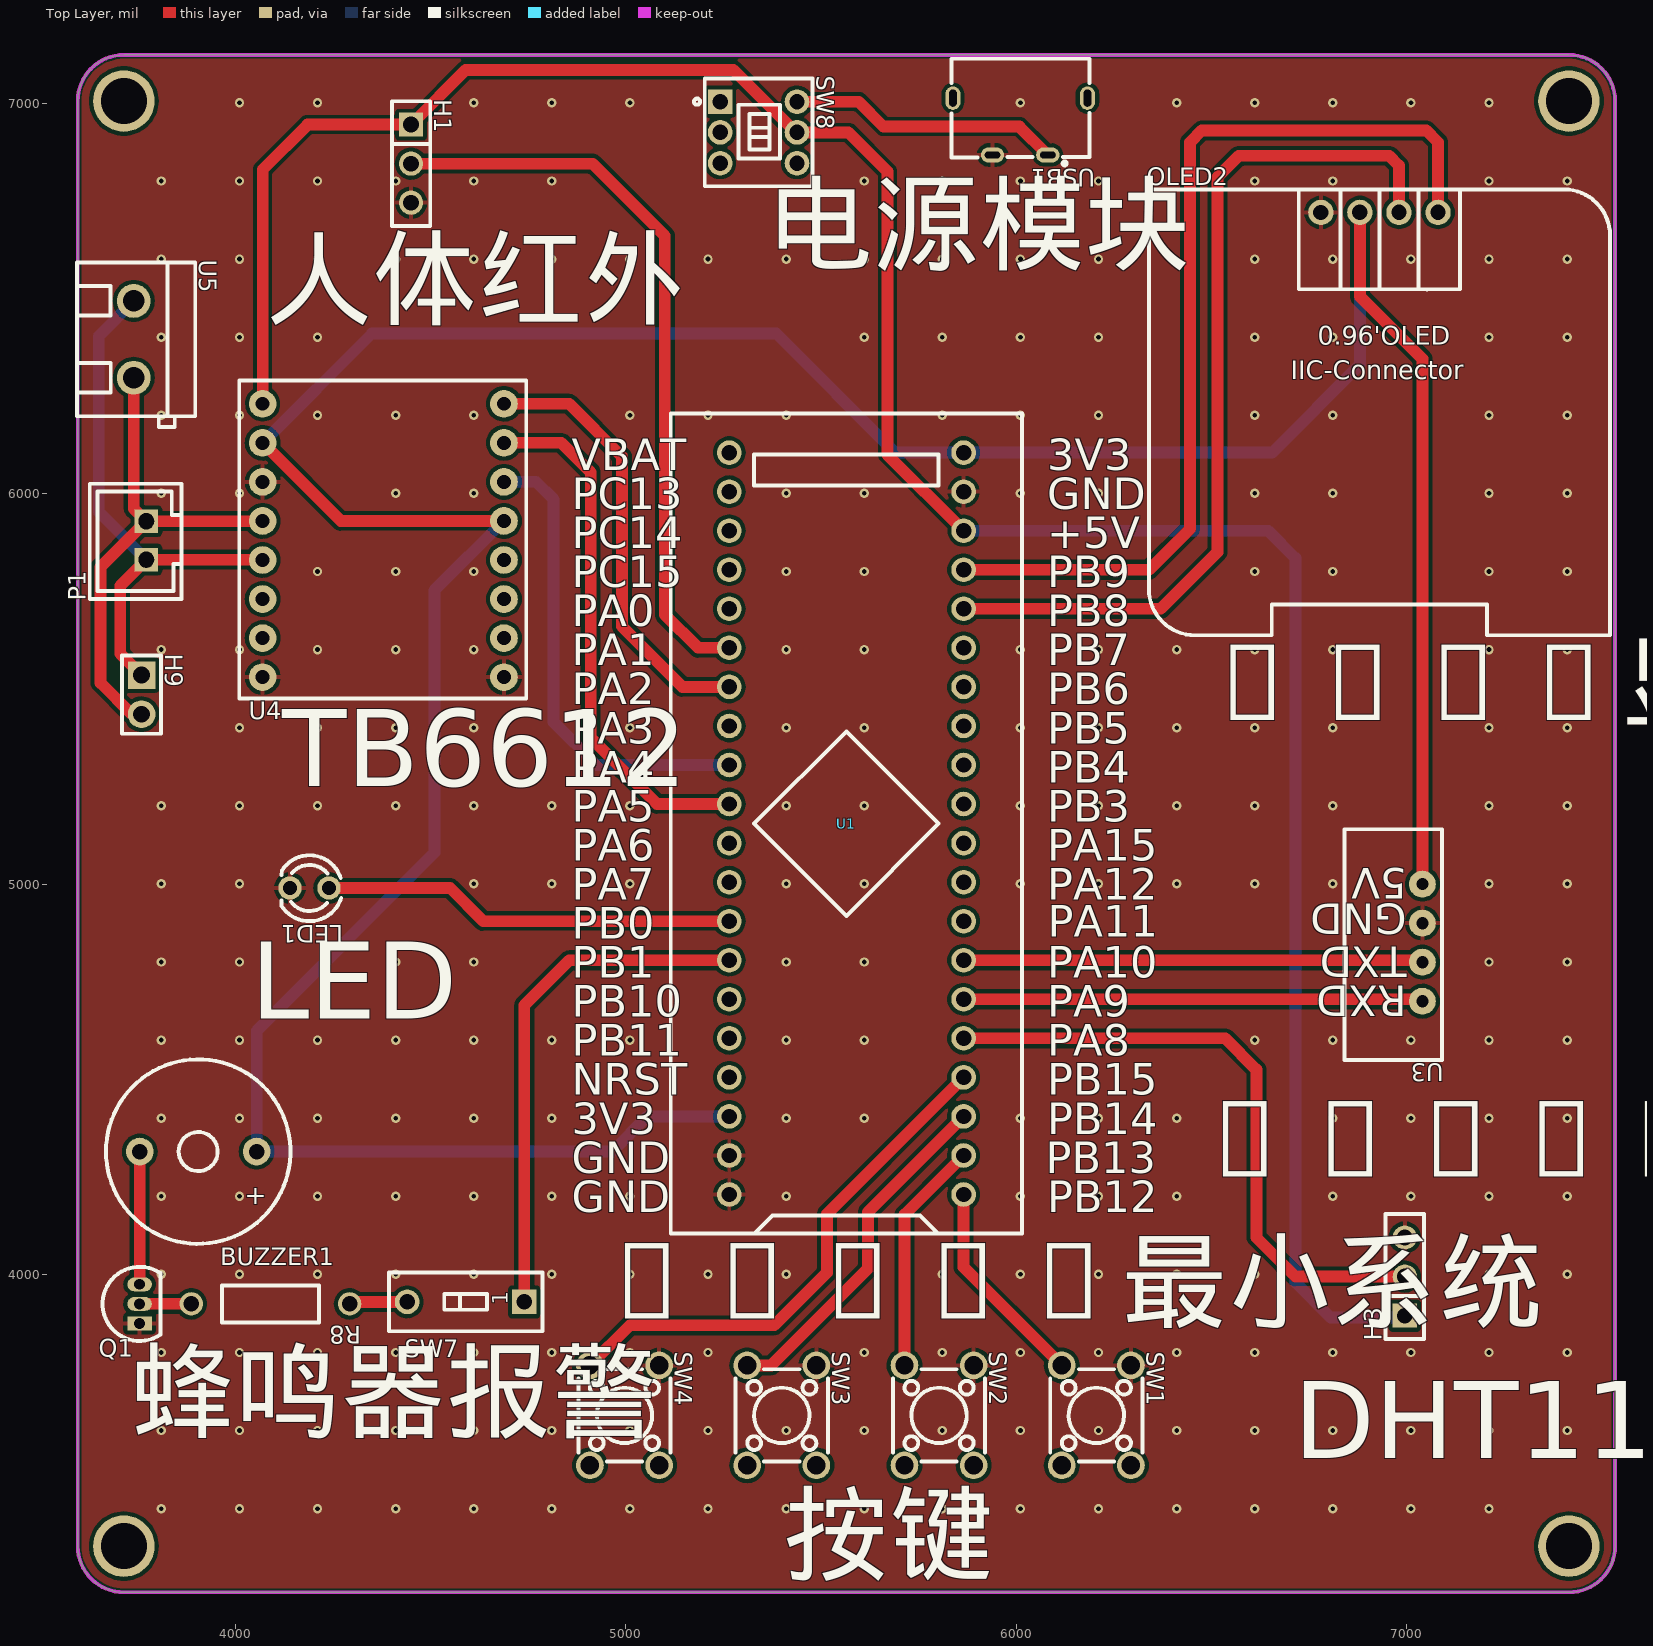
[diagram p0: Top Layer view]
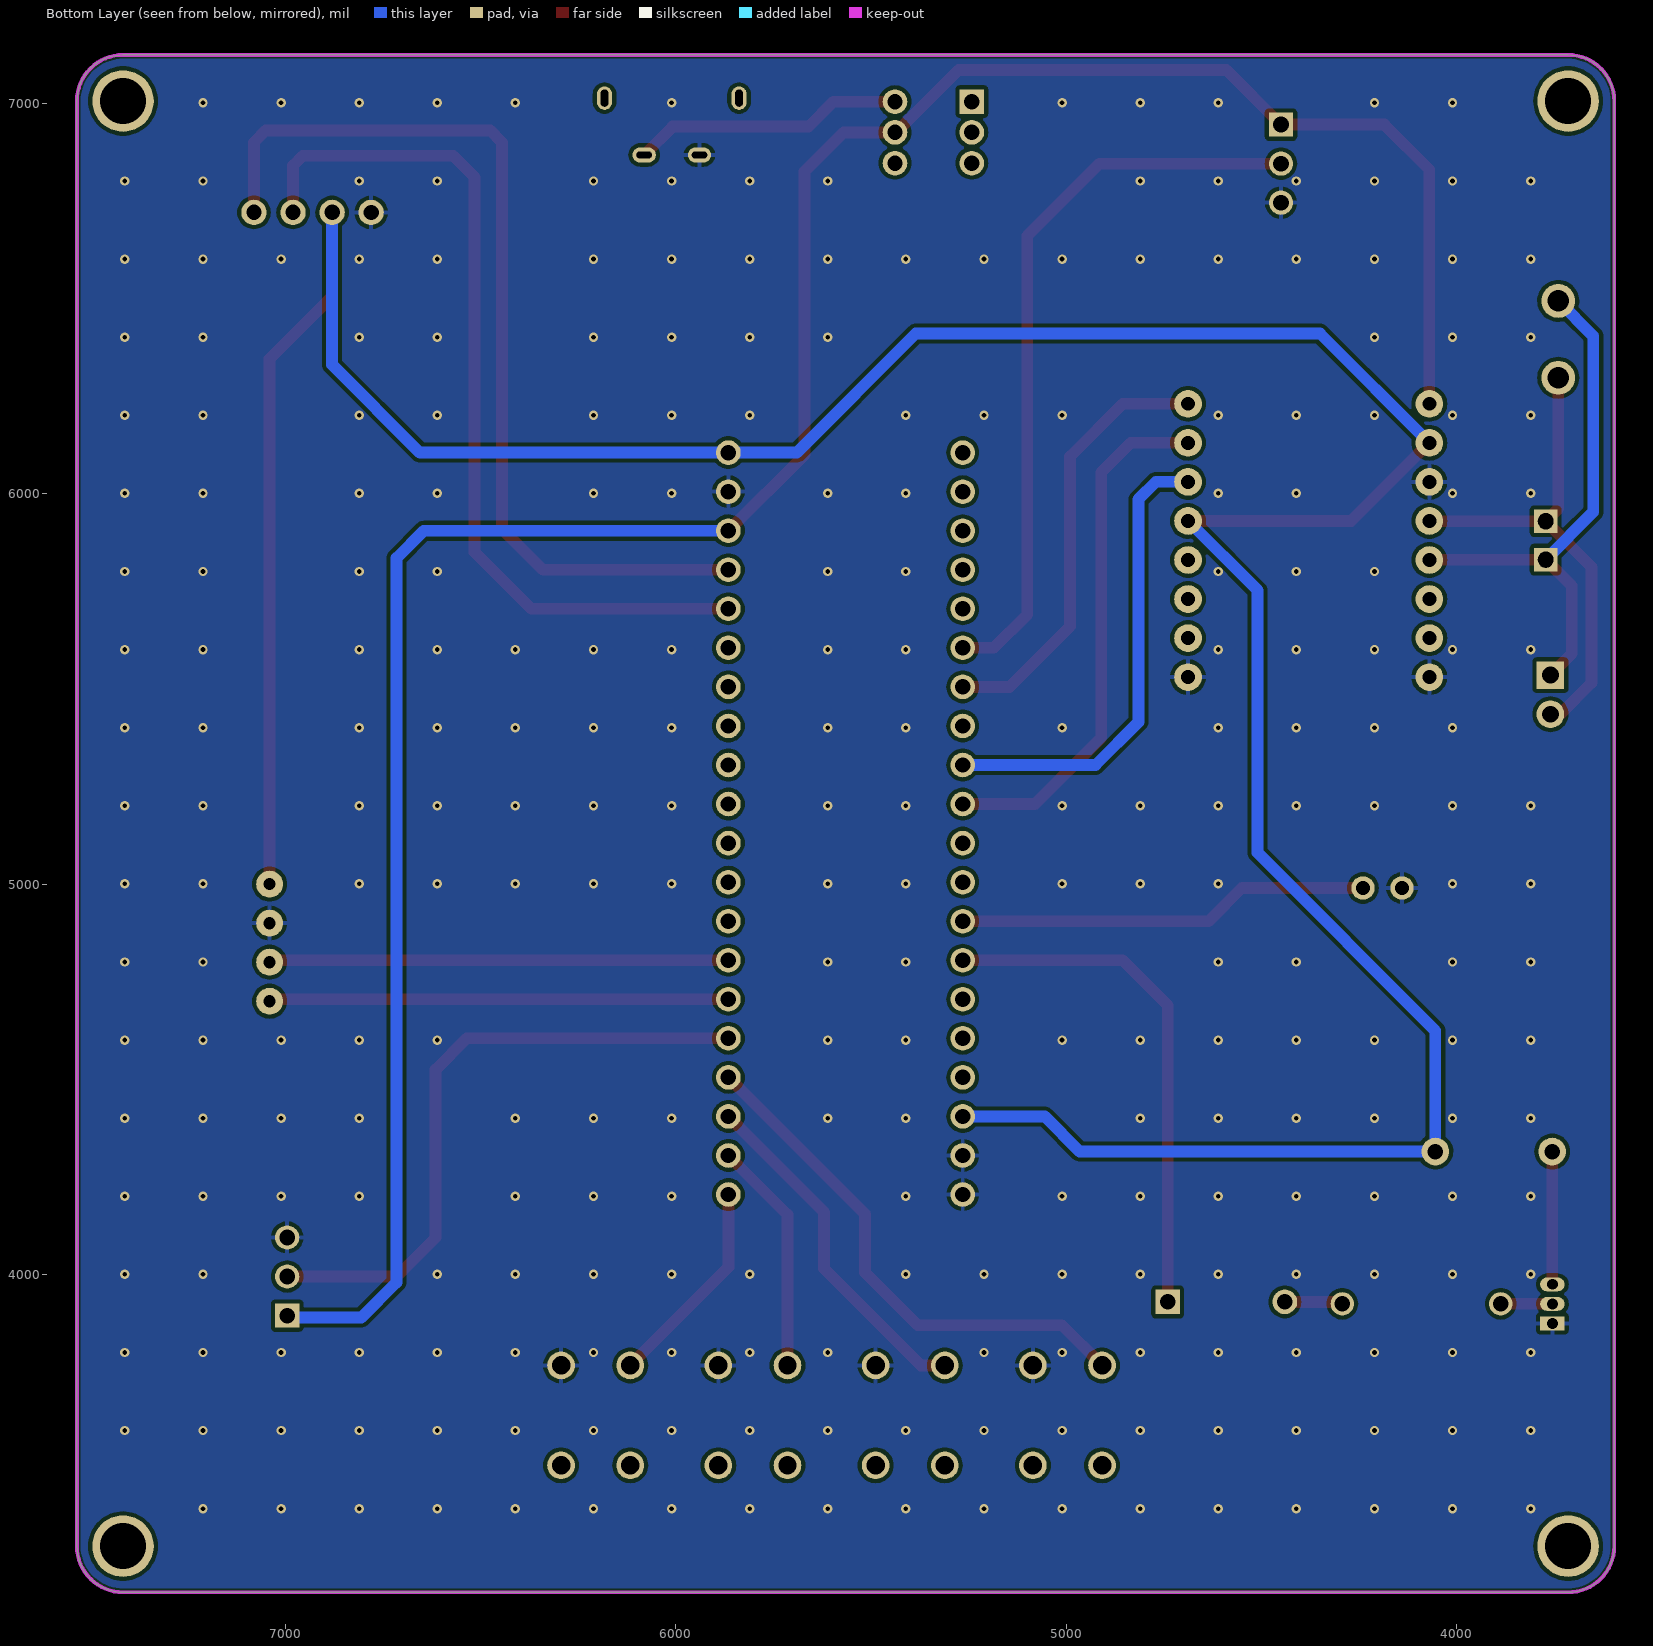
[diagram p1: Bottom Layer view, seen from below]
# Altium PCB MISC51405.pcbdoc
Units mil, origin at the board's own origin, x right, y up, seen from the top; angles counter-clockwise.
Board outline 3937.01 x 3937.01 mil, 2 copper layers (Top Layer, Bottom Layer), stack 62.206 mil thick; 20 components, 24 nets, 117 pads, 271 vias.

## Layer stack, top to bottom
Top Solder Mask Layer: solder mask 0.394, Dk 3.3
Top Layer: signal copper 1.379
Dielectric1: surface 59.449, FR4, Dk 4.5
Bottom Layer: signal copper 1.378
Bottom Solder Mask Layer: solder mask 0.394, Dk 3.3

## Board outline
3714.61,7123.5 ccw(c3714.61,7005.39) 3596.5,7005.39 3596.5,3304.61 ccw(c3714.61,3304.61) 3714.61,3186.5 7415.39,3186.5 ccw(c7415.39,3304.61) 7533.5,3304.61 7533.5,7005.39 ccw(c7415.39,7005.39) 7415.39,7123.5 3714.61,7123.5

## Design rules (kind name [scope] priority, off if disabled: settings)
BoardOutlineClearance copperThickness2oz_1 [All] p2 off: genericclearance=7.99 ignorepadtopadclearanceinfootprint=FALSE except(0: Arc-SplitContinuation Track-SplitContinuation SMDPad-SplitContinuation THPad-SplitContinuation Via-SplitContinuation Fill-SplitContinuation Region-SplitContinuation Poly-SplitContinuation Text-SplitContinuation Hole-SplitContinuation; 5.98: Arc-CutoutEdge Track-CutoutEdge SMDPad-CutoutEdge THPad-CutoutEdge Via-CutoutEdge Text-CutoutEdge; 6.9: Hole-OutlineEdge Hole-CutoutEdge; 10: Poly-OutlineEdge Poly-CutoutEdge; 11.81: Arc-OutlineEdge Track-OutlineEdge SMDPad-OutlineEdge THPad-OutlineEdge Via-OutlineEdge Fill-OutlineEdge Region-OutlineEdge Text-OutlineEdge Fill-CutoutEdge Region-CutoutEdge)
BoardOutlineClearance Plane_innerPlane_1 [All] p4 off: genericclearance=4.02 ignorepadtopadclearanceinfootprint=FALSE except(0: Arc-SplitContinuation Track-SplitContinuation SMDPad-SplitContinuation THPad-SplitContinuation Via-SplitContinuation Fill-SplitContinuation Region-SplitContinuation Poly-SplitContinuation Text-SplitContinuation Hole-SplitContinuation; 5.98: Arc-CutoutEdge Track-CutoutEdge SMDPad-CutoutEdge THPad-CutoutEdge Via-CutoutEdge Text-CutoutEdge; 6.9: Hole-OutlineEdge Hole-CutoutEdge; 10: Poly-OutlineEdge Poly-CutoutEdge; 11.81: Arc-OutlineEdge Track-OutlineEdge SMDPad-OutlineEdge THPad-OutlineEdge Via-OutlineEdge Fill-OutlineEdge Region-OutlineEdge Text-OutlineEdge Fill-CutoutEdge Region-CutoutEdge)
BoardOutlineClearance Copper_copperRegion_1 [All] p6 off: genericclearance=4.02 ignorepadtopadclearanceinfootprint=FALSE except(0: Arc-SplitContinuation Track-SplitContinuation SMDPad-SplitContinuation THPad-SplitContinuation Via-SplitContinuation Fill-SplitContinuation Region-SplitContinuation Poly-SplitContinuation Text-SplitContinuation Hole-SplitContinuation; 5.98: Arc-CutoutEdge Track-CutoutEdge SMDPad-CutoutEdge THPad-CutoutEdge Via-CutoutEdge Text-CutoutEdge; 6.9: Hole-OutlineEdge Hole-CutoutEdge; 10: Poly-OutlineEdge Poly-CutoutEdge; 11.81: Arc-OutlineEdge Track-OutlineEdge SMDPad-OutlineEdge THPad-OutlineEdge Via-OutlineEdge Fill-OutlineEdge Region-OutlineEdge Text-OutlineEdge Fill-CutoutEdge Region-CutoutEdge)
BoardOutlineClearance Copper_copperRegion_copperThickness1oz_1 [All] p8 off: genericclearance=4.02 ignorepadtopadclearanceinfootprint=FALSE except(0: Arc-SplitContinuation Track-SplitContinuation SMDPad-SplitContinuation THPad-SplitContinuation Via-SplitContinuation Fill-SplitContinuation Region-SplitContinuation Poly-SplitContinuation Text-SplitContinuation Hole-SplitContinuation; 5.98: Arc-CutoutEdge Track-CutoutEdge SMDPad-CutoutEdge THPad-CutoutEdge Via-CutoutEdge Text-CutoutEdge; 6.9: Hole-OutlineEdge Hole-CutoutEdge; 10: Poly-OutlineEdge Poly-CutoutEdge; 11.81: Arc-OutlineEdge Track-OutlineEdge SMDPad-OutlineEdge THPad-OutlineEdge Via-OutlineEdge Fill-OutlineEdge Region-OutlineEdge Text-OutlineEdge Fill-CutoutEdge Region-CutoutEdge)
BoardOutlineClearance Copper_copperRegion_Copper_copperRegion_1 [All] p10 off: genericclearance=4.02 ignorepadtopadclearanceinfootprint=FALSE except(0: Arc-SplitContinuation Track-SplitContinuation SMDPad-SplitContinuation THPad-SplitContinuation Via-SplitContinuation Fill-SplitContinuation Region-SplitContinuation Poly-SplitContinuation Text-SplitContinuation Hole-SplitContinuation; 5.98: Arc-CutoutEdge Track-CutoutEdge SMDPad-CutoutEdge THPad-CutoutEdge Via-CutoutEdge Text-CutoutEdge; 6.9: Hole-OutlineEdge Hole-CutoutEdge; 10: Poly-OutlineEdge Poly-CutoutEdge; 11.81: Arc-OutlineEdge Track-OutlineEdge SMDPad-OutlineEdge THPad-OutlineEdge Via-OutlineEdge Fill-OutlineEdge Region-OutlineEdge Text-OutlineEdge Fill-CutoutEdge Region-CutoutEdge)
BoardOutlineClearance copperThickness1oz_1 [All] p12: genericclearance=4.02 ignorepadtopadclearanceinfootprint=FALSE except(0: Arc-SplitContinuation Track-SplitContinuation SMDPad-SplitContinuation THPad-SplitContinuation Via-SplitContinuation Fill-SplitContinuation Region-SplitContinuation Poly-SplitContinuation Text-SplitContinuation Hole-SplitContinuation; 5.98: Arc-CutoutEdge Track-CutoutEdge SMDPad-CutoutEdge THPad-CutoutEdge Via-CutoutEdge Text-CutoutEdge; 6.9: Hole-OutlineEdge Hole-CutoutEdge; 10: Poly-OutlineEdge Poly-CutoutEdge; 11.81: Arc-OutlineEdge Track-OutlineEdge SMDPad-OutlineEdge THPad-OutlineEdge Via-OutlineEdge Fill-OutlineEdge Region-OutlineEdge Text-OutlineEdge Fill-CutoutEdge Region-CutoutEdge)
Clearance copperThickness2oz [All] p1 off: gap=7.99 ignorepadtopadclearanceinfootprint=FALSE except(5.98: SMDPad-Track SMDPad-SMDPad THPad-Track SMDPad-THPad THPad-THPad Track-Via SMDPad-Via THPad-Via Via-Via Fill-SMDPad Region-SMDPad Fill-THPad Region-THPad Fill-Via Region-Via Fill-Fill Fill-Region Region-Region Arc-Track Arc-SMDPad Arc-THPad Arc-Via Fill-Arc Region-Arc Arc-Arc Text-Track SMDPad-Text Text-THPad Text-Via Fill-Text Region-Text Arc-Text Text-Text; 6.9: Hole-Track Hole-SMDPad Hole-THPad Hole-Via Fill-Hole Region-Hole Hole-Arc Hole-Text; 10: Poly-Track Poly-SMDPad Poly-THPad Poly-Via Poly-Fill Poly-Region Poly-Poly Poly-Arc Poly-Text Poly-Hole; 11.81: Fill-Track Region-Track)
Clearance Plane_innerPlane [All] p3 off: gap=4.02 ignorepadtopadclearanceinfootprint=FALSE except(5.98: SMDPad-Track SMDPad-SMDPad THPad-Track SMDPad-THPad THPad-THPad Track-Via SMDPad-Via THPad-Via Via-Via Fill-SMDPad Region-SMDPad Fill-THPad Region-THPad Fill-Via Region-Via Fill-Fill Fill-Region Region-Region Arc-Track Arc-SMDPad Arc-THPad Arc-Via Fill-Arc Region-Arc Arc-Arc Text-Track SMDPad-Text Text-THPad Text-Via Fill-Text Region-Text Arc-Text Text-Text; 6.9: Hole-Track Hole-SMDPad Hole-THPad Hole-Via Fill-Hole Region-Hole Hole-Arc Hole-Text; 10: Poly-Track Poly-SMDPad Poly-THPad Poly-Via Poly-Fill Poly-Region Poly-Poly Poly-Arc Poly-Text Poly-Hole; 11.81: Fill-Track Region-Track)
Clearance Copper_copperRegion [All] p5 off: gap=4.02 ignorepadtopadclearanceinfootprint=FALSE except(5.98: SMDPad-Track SMDPad-SMDPad THPad-Track SMDPad-THPad THPad-THPad Track-Via SMDPad-Via THPad-Via Via-Via Fill-SMDPad Region-SMDPad Fill-THPad Region-THPad Fill-Via Region-Via Fill-Fill Fill-Region Region-Region Arc-Track Arc-SMDPad Arc-THPad Arc-Via Fill-Arc Region-Arc Arc-Arc Text-Track SMDPad-Text Text-THPad Text-Via Fill-Text Region-Text Arc-Text Text-Text; 6.9: Hole-Track Hole-SMDPad Hole-THPad Hole-Via Fill-Hole Region-Hole Hole-Arc Hole-Text; 10: Poly-Track Poly-SMDPad Poly-THPad Poly-Via Poly-Fill Poly-Region Poly-Poly Poly-Arc Poly-Text Poly-Hole; 11.81: Fill-Track Region-Track)
Clearance Copper_copperRegion_copperThickness1oz [All] p7 off: gap=4.02 ignorepadtopadclearanceinfootprint=FALSE except(5.98: SMDPad-Track SMDPad-SMDPad THPad-Track SMDPad-THPad THPad-THPad Track-Via SMDPad-Via THPad-Via Via-Via Fill-SMDPad Region-SMDPad Fill-THPad Region-THPad Fill-Via Region-Via Fill-Fill Fill-Region Region-Region Arc-Track Arc-SMDPad Arc-THPad Arc-Via Fill-Arc Region-Arc Arc-Arc Text-Track SMDPad-Text Text-THPad Text-Via Fill-Text Region-Text Arc-Text Text-Text; 6.9: Hole-Track Hole-SMDPad Hole-THPad Hole-Via Fill-Hole Region-Hole Hole-Arc Hole-Text; 10: Poly-Track Poly-SMDPad Poly-THPad Poly-Via Poly-Fill Poly-Region Poly-Poly Poly-Arc Poly-Text Poly-Hole; 11.81: Fill-Track Region-Track)
Clearance Copper_copperRegion_Copper_copperRegion [All] p9 off: gap=4.02 ignorepadtopadclearanceinfootprint=FALSE except(5.98: SMDPad-Track SMDPad-SMDPad THPad-Track SMDPad-THPad THPad-THPad Track-Via SMDPad-Via THPad-Via Via-Via Fill-SMDPad Region-SMDPad Fill-THPad Region-THPad Fill-Via Region-Via Fill-Fill Fill-Region Region-Region Arc-Track Arc-SMDPad Arc-THPad Arc-Via Fill-Arc Region-Arc Arc-Arc Text-Track SMDPad-Text Text-THPad Text-Via Fill-Text Region-Text Arc-Text Text-Text; 6.9: Hole-Track Hole-SMDPad Hole-THPad Hole-Via Fill-Hole Region-Hole Hole-Arc Hole-Text; 10: Poly-Track Poly-SMDPad Poly-THPad Poly-Via Poly-Fill Poly-Region Poly-Poly Poly-Arc Poly-Text Poly-Hole; 11.81: Fill-Track Region-Track)
Clearance copperThickness1oz [All] p11: gap=4.02 ignorepadtopadclearanceinfootprint=FALSE except(5.98: SMDPad-Track SMDPad-SMDPad THPad-Track SMDPad-THPad THPad-THPad Track-Via SMDPad-Via THPad-Via Via-Via Fill-SMDPad Region-SMDPad Fill-THPad Region-THPad Fill-Via Region-Via Fill-Fill Fill-Region Region-Region Arc-Track Arc-SMDPad Arc-THPad Arc-Via Fill-Arc Region-Arc Arc-Arc Text-Track SMDPad-Text Text-THPad Text-Via Fill-Text Region-Text Arc-Text Text-Text; 6.9: Hole-Track Hole-SMDPad Hole-THPad Hole-Via Fill-Hole Region-Hole Hole-Arc Hole-Text; 10: Poly-Track Poly-SMDPad Poly-THPad Poly-Via Poly-Fill Poly-Region Poly-Poly Poly-Arc Poly-Text Poly-Hole; 11.81: Fill-Track Region-Track)
DiffPairsRouting differentialPair [All] p1: maxlimit=6 minlimit=6 mostfreqgap=6 toplayer_minwidth=5 toplayer_prefwidth=10 toplayer_maxwidth=100 toplayer_mingap=6 toplayer_prefgap=6 toplayer_maxgap=6 bottomlayer_minwidth=5 bottomlayer_prefwidth=10 bottomlayer_maxwidth=100 bottomlayer_mingap=6 bottomlayer_prefgap=6 bottomlayer_maxgap=6 maxuncoupledlength=10
HoleToHoleClearance otherClearance [All] p1: gap=11.81 allowstackedmicrovias=TRUE
Length netLength [All] p1: minlimit=0 maxlimit=0
PasteMaskExpansion pasteMaskExpansion [All] p1: expansion=0
PlaneConnect innerPlane [All] p1: planeconnectstyle=Relief reliefexpansion=20 reliefentries=4 reliefconductorwidth=10 reliefairgap=10
PolygonConnect copperRegion_copperThickness1oz [All] p1 off: connectstyle=Relief reliefconductorwidth=10 reliefentries=4 polygonreliefangle="90 Angle" airgapwidth=10 via.connectstyle=Relief via.reliefconductorwidth=10 via.reliefentries=4 via.polygonreliefangle="90 Angle" via.airgapwidth=10
PolygonConnect copperRegion_Copper_copperRegion [All] p2 off: connectstyle=Relief reliefconductorwidth=10 reliefentries=4 polygonreliefangle="90 Angle" airgapwidth=10 via.connectstyle=Relief via.reliefconductorwidth=10 via.reliefentries=4 via.polygonreliefangle="90 Angle" via.airgapwidth=10
PolygonConnect copperRegion [All] p3: connectstyle=Relief reliefconductorwidth=10 reliefentries=4 polygonreliefangle="90 Angle" airgapwidth=10 via.connectstyle=Relief via.reliefconductorwidth=10 via.reliefentries=4 via.polygonreliefangle="90 Angle" via.airgapwidth=10
RoutingVias viaSize [All] p1: holewidth=12.01 width=24.02 viastyle="Through Hole" minholewidth=11.81 minwidth=19.68 maxholewidth=248.03 maxwidth=393.7
SolderMaskExpansion solderMaskExpansion [IsVia] p1: expansion=-1000 istentingtop=TRUE
SolderMaskExpansion solderMaskExpansion [All] p2: expansion=2 istentingtop=FALSE
Width copperThickness2oz_2 [All] p1 off: maxlimit=100 minlimit=8 preferedwidth=10
Width copperThickness1oz_2 [All] p2: maxlimit=100 minlimit=5 preferedwidth=10

## Components (designator, comment, footprint, x,y, rotation, side; value= is the part's Value field where it differs from the comment)
BUZZER1 "2.3kHz" BUZ-TH_BD12.0-P7.60-D0.6-FD 3905,4315 r180 top
H1 "" HDR-TH_3P-P2.54-V-F 4450,6845 r270 top
H3 "" HDR-TH_3P-P2.54-V-F 6995,3995 r90 top
H9 "" HDR-TH_2P-P2.54-V-M-1 3760,5485 r270 top
LED1 "" LED_TH-3mm 4190,4990 r180 top
OLED2 "" 0.96OLED_4P 6930,6720 r0 top
P1 "XH2.54直插座-2P" CONN-TH_XH2.54-2P 3772.17,5880.14 r90 top
Q1 "" S8050_TO_92 3755,3925 r90 top
R8 "10kΩ" Res_1/4W 4090,3925 r180 top
SW1 "" SW-TH_4P-L6.0-W6.0-P4.50-LS6.5 6205,3639.42 r270 top
SW2 "" SW-TH_4P-L6.0-W6.0-P4.50-LS6.5 5802.24,3639.42 r270 top
SW3 "" SW-TH_4P-L6.0-W6.0-P4.50-LS6.5 5399.48,3639.42 r270 top
SW4 "" SW-TH_4P-L6.0-W6.0-P4.50-LS6.5 4996.72,3639.42 r270 top
SW7 "拨码开关1位" SW-TH_2P-L3.9-W9.9-P2.54-LS7.6 4590,3930 r180 top
SW8 "TK-6700-1" SW-TH_TK-6700-1 5340,6925 r270 top
U1 "STM32F103C8T6-Card" CONN-TH_L53.3-W22.9_STM32F103C8T6-CARD 5565,5155 r90 top
U3 "" BT04-A 7040,4700 r180 top
U4 "" tb6612 4070,6230 r0 top
U5 "KF301-5.0-2P" CONN-TH_P5.00_KF301-5.0-2P 3740,6395 r270 top
USB1 "KH-TYPE-C-2P" USB-SMD_KH-TYPE-C-2P 6010,6940 r180 top

## Footprints (in the part's own frame and the unit in brackets; to place one, negate y for a bottom-side part, rotate by r counter-clockwise, add the part's x,y. Pads: shape width x height; smd on the part's side, far side on the other; paste and mask are expansions set on the pad)
0.96OLED_4P [mm]
  round 1.65 hole 1 copper offset 0,0: 1(-3.81,-0.001) 2(-1.27,0.002) 3(1.27,0.002) 4(3.81,0.002)
  silkscreen extent -15,-27.5 15,1.5
BT04-A [mm]
  round 1.75 hole 0.8: 1(0,0) 2(0,-2.54) 3(0,-5.08) 4(0,-7.62)
  silkscreen extent -1.27,-11.19 5.08,3.81
BUZ-TH_BD12.0-P7.60-D0.6-FD [mm]
  round 1.8 hole 1: 1(-3.8,0) 2(3.8,0)
  silkscreen extent -6,-6 6,6
CONN-TH_L53.3-W22.9_STM32F103C8T6-CARD [mm]
  round 1.6 hole 1: 1(-24.13,-7.62) 2(-21.59,-7.62) 3(-19.05,-7.62) 4(-16.51,-7.62) 5(-13.97,-7.62) 6(-11.43,-7.62) 7(-8.89,-7.62) 8(-6.35,-7.62) 9(-3.81,-7.62) 10(-1.27,-7.62) 11(1.27,-7.62) 12(3.81,-7.62) 13(6.35,-7.62) 14(8.89,-7.62) 15(11.43,-7.62) 16(13.97,-7.62) 17(16.51,-7.62) 18(19.05,-7.62) 19(21.59,-7.62) 20(24.13,-7.62) 21(24.13,7.62) 22(21.59,7.62) 23(19.05,7.62) 24(16.51,7.62) 25(13.97,7.62) 26(11.43,7.62) 27(8.89,7.62) 28(6.35,7.62) 29(3.81,7.62) 30(1.27,7.62) 31(-1.27,7.62) 32(-3.81,7.62) 33(-6.35,7.62) 34(-8.89,7.62) 35(-11.43,7.62) 36(-13.97,7.62) 37(-16.51,7.62) 38(-19.05,7.62) 39(-21.59,7.62) 40(-24.13,7.62)
  silkscreen extent -26.67,-11.43 26.67,11.43
CONN-TH_P5.00_KF301-5.0-2P [mm]
  round 2.2 hole 1.4 paste+0 mask+0.05: 1(-2.5,0) 2(2.5,0)
  silkscreen extent -5,-3.7 5.71,4
CONN-TH_XH2.54-2P [mil]
  rect 60x60 hole 39.37 slot 41.34 at 0 deg paste+0 mask+1.97: 1(-49.22,0) 2(49.21,0)
  silkscreen extent -150,-90 145,145
HDR-TH_2P-P2.54-V-M-1 [mm]
  rect 1.8x1.8 hole 1.1: 1(-1.27,0)
  round 1.8 hole 1.1: 2(1.27,0)
  silkscreen extent -2.54,-1.27 2.54,1.27
HDR-TH_3P-P2.54-V-F [mil]
  rect 62x62 hole 40.16: 1(-100,0)
  round 62 hole 40.16: 2(0,0) 3(100,0)
  silkscreen extent -160,-49 160,49
LED_TH-3mm [mil]
  round 60 hole 36 paste+0 mask+2: 1(-50,0) 2(50,0)
  silkscreen extent -81,-84 72,85
Res_1/4W [mil]
  round 60 hole 39.37 paste+0 mask+2: 1(-202.76,0) 2(202.76,0)
  silkscreen extent -124,-47 124,47
S8050_TO_92 [mil]
  rect 35.4x63 hole 27.6 paste+0 mask+2: 1(-50,0)
  oval 35.4x63 hole 27.6 paste+0 mask+2: 2(0,0) 3(50,0)
  silkscreen extent -95,-53 95,95
SW-TH_2P-L3.9-W9.9-P2.54-LS7.6 [mm]
  rect 1.6x1.6 hole 1 paste+0 mask+0.05: 1(-3.81,0)
  round 1.6 hole 1 paste+0 mask+0.05: 2(3.81,0)
  silkscreen extent -5,-1.91 5,1.91
SW-TH_4P-L6.0-W6.0-P4.50-LS6.5 [mm]
  round 1.8 hole 1.2: 1(-3.25,2.25) 2(3.25,2.25) 3(-3.25,-2.25) 4(3.25,-2.25)
  silkscreen extent -3,-3 3,3
SW-TH_TK-6700-1 [mm]
  rect 1.6x1.6 hole 1 paste+0 mask+0.051: 1(-2,-2.5)
  round 1.6 hole 1 paste+0 mask+0.051: 2(0,-2.5) 3(2,-2.5)
  round 1.6 hole 1 copper offset 0,0 paste+0 mask+0.051: 4(-2,2.5) 5(0,2.5) 6(2,2.5)
  silkscreen extent -3.5,-4.2 3.5,3.5
tb6612 [mm]
  round 1.8 hole 0.9: 1(0,0) 2(0,-2.54) 3(0,-5.08) 4(0,-7.62) 5(0,-10.16) 6(0,-12.7) 7(0,-15.24) 8(0,-17.78) 9(15.697,-17.78) 10(15.697,-15.24) 11(15.697,-12.7) 12(15.697,-10.16) 13(15.697,-7.62) 14(15.697,-5.08) 15(15.697,-2.54) 16(15.697,0)
  silkscreen extent -1.52,-19.18 17.14,1.52
USB-SMD_KH-TYPE-C-2P [mm]
  oval 1.524x1 hole 0.45 slot 1 at 0 deg paste+0 mask+0.05: 1(-1.8,1.85) 2(1.8,1.85)
  oval 1x1.524 hole 0.5 slot 1.1 at 90 deg paste+0 mask+0.05: 3(4.375,-1.85) 4(-4.375,-1.85)
  silkscreen extent -4.5,-4.41 4.46,2.53

## Free pads (board coordinates)
  round 157.48 hole 118.11: 1(3714.61,7005.39) 1(3714.61,3304.61) 1(7415.39,7005.39) 1(7415.39,3304.61)

## Via types
v1: diameter 24.02, hole 12, Top Layer to Bottom Layer, 271 vias

## Nets (pads, with @x,y where several pads share a name; then routed paths per layer and width w, separated by ;. In a path a pad name is that pad's centre, name@x,y a point inside that pad or via, vN(x,y) a via of type N, cw(c..) or ccw(c..) an arc to the next point about the centre after c; other vN are vias at no path point)
$1N17271: Q1.2 R8.2 | length 132.2
  Top Layer w30: Q1.2 R8.2
$1N17275: BUZZER1.2 Q1.3 | length 340.2
  Top Layer w30: Q1.3 3755,4314.6 BUZZER1.2
$1N17276: R8.1 SW7.2 | length 149.3
  Top Layer w30: R8.1 4297.76,3930 SW7.2
+5V: H1.1 H3.1 SW8.5 U1.18 U4.1 | length 6467.4
  Top Layer w30: U4.1 4070,6830 4185,6945 H1.1 4590,7085 5275,7085 5435,6925 SW8.5 5570,6925 5670,6825 5670,6100 U1.18
  Bottom Layer w30: U1.18 6645,5905 6715,5835 6715,3980 6805,3890 6990,3890 H3.1
AIN1: U1.29 U4.14 | length 1211.2
  Bottom Layer w30: U4.14 4770,6030 4815,5985 4815,5415 4925,5305 U1.29
AIN2: U1.30 U4.15 | length 1358.5
  Top Layer w30: U4.15 4835,6130 4910,6055 4910,5375 5080,5205 U1.30
BEEP: SW7.1 U1.34 | length 1332.6
  Top Layer w30: SW7.1 4740,4690 4855,4805 U1.34
DHT11: H3.2 U1.5 | length 1634.6
  Top Layer w30: U1.5 6535,4605 6615,4525 6615,4095 6715,3995 H3.2
GND: H1.3 H3.3 LED1.2 OLED2.1 Q1.1 SW1.1 SW2.1 SW3.1 SW4.1 U1.19 U1.39 U1.40 U3.3 U4.3 U4.8 U4.9 USB1.2
  other v1: 3810.6,3400.6 4010.6,3400.6 4210.6,3400.6 4410.6,3400.6 4610.6,3400.6 4810.6,3400.6 5010.6,3400.6 5210.6,3400.6 5410.6,3400.6 5610.6,3400.6 5810.6,3400.6 6010.6,3400.6 6210.6,3400.6 6410.6,3400.6 6610.6,3400.6 6810.6,3400.6 7010.6,3400.6 7210.6,3400.6 3810.6,3600.6 4010.6,3600.6 4210.6,3600.6 4410.6,3600.6 4610.6,3600.6 4810.6,3600.6 5010.6,3600.6 5210.6,3600.6 5410.6,3600.6 5610.6,3600.6 5810.6,3600.6 6010.6,3600.6 6210.6,3600.6 6410.6,3600.6 6610.6,3600.6 6810.6,3600.6 7010.6,3600.6 7210.6,3600.6 7410.6,3600.6 3810.6,3800.6 4010.6,3800.6 4210.6,3800.6 4410.6,3800.6 4610.6,3800.6 4810.6,3800.6 5010.6,3800.6 5210.6,3800.6 5610.6,3800.6 5810.6,3800.6 6010.6,3800.6 6210.6,3800.6 6410.6,3800.6 6610.6,3800.6 6810.6,3800.6 7010.6,3800.6 7210.6,3800.6 7410.6,3800.6 3810.6,4000.6 4010.6,4000.6 4210.6,4000.6 4410.6,4000.6 4610.6,4000.6 4810.6,4000.6 5010.6,4000.6 5210.6,4000.6 5410.6,4000.6 5810.6,4000.6 6010.6,4000.6 6210.6,4000.6 6410.6,4000.6 6610.6,4000.6 7210.6,4000.6 7410.6,4000.6 3810.6,4200.6 4010.6,4200.6 4210.6,4200.6 4410.6,4200.6 4610.6,4200.6 4810.6,4200.6 5010.6,4200.6 5410.6,4200.6 6010.6,4200.6 6210.6,4200.6 6410.6,4200.6 6810.6,4200.6 7010.6,4200.6 7210.6,4200.6 7410.6,4200.6 3810.6,4400.6 4010.6,4400.6 4210.6,4400.6 4410.6,4400.6 4610.6,4400.6 4810.6,4400.6 5410.6,4400.6 5610.6,4400.6 6010.6,4400.6 6210.6,4400.6 6410.6,4400.6 6810.6,4400.6 7010.6,4400.6 7210.6,4400.6 7410.6,4400.6 3810.6,4600.6 4010.6,4600.6 4210.6,4600.6 4410.6,4600.6 4610.6,4600.6 4810.6,4600.6 5010.6,4600.6 5410.6,4600.6 5610.6,4600.6 6610.6,4600.6 6810.6,4600.6 7010.6,4600.6 7210.6,4600.6 7410.6,4600.6 3810.6,4800.6 4010.6,4800.6 4410.6,4800.6 4610.6,4800.6 5410.6,4800.6 5610.6,4800.6 7210.6,4800.6 7410.6,4800.6 3810.6,5000.6 4010.6,5000.6 4610.6,5000.6 4810.6,5000.6 5010.6,5000.6 5410.6,5000.6 5610.6,5000.6 6010.6,5000.6 6210.6,5000.6 6410.6,5000.6 6610.6,5000.6 6810.6,5000.6 7210.6,5000.6 7410.6,5000.6 3810.6,5200.6 4010.6,5200.6 4210.6,5200.6 4410.6,5200.6 4610.6,5200.6 4810.6,5200.6 5010.6,5200.6 5410.6,5200.6 5610.6,5200.6 6010.6,5200.6 6210.6,5200.6 6410.6,5200.6 6610.6,5200.6 6810.6,5200.6 7210.6,5200.6 7410.6,5200.6 4010.6,5400.6 4210.6,5400.6 4410.6,5400.6 4610.6,5400.6 5010.6,5400.6 5410.6,5400.6 5610.6,5400.6 6010.6,5400.6 6210.6,5400.6 6410.6,5400.6 6610.6,5400.6 6810.6,5400.6 7210.6,5400.6 7410.6,5400.6 3810.6,5600.6 4010.6,5600.6 4210.6,5600.6 4410.6,5600.6 4610.6,5600.6 5410.6,5600.6 5610.6,5600.6 6010.6,5600.6 6210.6,5600.6 6410.6,5600.6 6610.6,5600.6 6810.6,5600.6 7210.6,5600.6 7410.6,5600.6 4210.6,5800.6 4410.6,5800.6 4610.6,5800.6 5410.6,5800.6 5610.6,5800.6 6610.6,5800.6 6810.6,5800.6 7210.6,5800.6 7410.6,5800.6 3810.6,6000.6 4010.6,6000.6 4410.6,6000.6 4610.6,6000.6 5410.6,6000.6 5610.6,6000.6 6010.6,6000.6 6210.6,6000.6 6610.6,6000.6 6810.6,6000.6 7210.6,6000.6 7410.6,6000.6 3810.6,6200.6 4010.6,6200.6 4210.6,6200.6 4410.6,6200.6 4610.6,6200.6 5010.6,6200.6 5210.6,6200.6 5410.6,6200.6 5810.6,6200.6 6010.6,6200.6 6210.6,6200.6 6610.6,6200.6 6810.6,6200.6 7210.6,6200.6 7410.6,6200.6 3810.6,6400.6 4010.6,6400.6 4210.6,6400.6 5610.6,6400.6 5810.6,6400.6 6010.6,6400.6 6210.6,6400.6 6610.6,6400.6 6810.6,6400.6 7210.6,6400.6 7410.6,6400.6 3810.6,6600.6 4010.6,6600.6 4210.6,6600.6 4410.6,6600.6 4610.6,6600.6 4810.6,6600.6 5010.6,6600.6 5210.6,6600.6 5410.6,6600.6 5610.6,6600.6 5810.6,6600.6 6010.6,6600.6 6210.6,6600.6 6610.6,6600.6 6810.6,6600.6 7010.6,6600.6 7210.6,6600.6 7410.6,6600.6 3810.6,6800.6 4010.6,6800.6 4210.6,6800.6 4410.6,6800.6 4610.6,6800.6 4810.6,6800.6 5610.6,6800.6 5810.6,6800.6 6010.6,6800.6 6210.6,6800.6 6610.6,6800.6 6810.6,6800.6 7210.6,6800.6 7410.6,6800.6 4010.6,7000.6 4210.6,7000.6 4610.6,7000.6 4810.6,7000.6 5010.6,7000.6 6010.6,7000.6 6410.6,7000.6 6610.6,7000.6 6810.6,7000.6 7010.6,7000.6 7210.6,7000.6
H+: H9.2 P1.2 U4.4 U5.2 | length 1279.7
  Top Layer w30: U5.2 3740,5961.53 P1.2 ; H9.2 3735,5435 3655,5515 3655,5812.18 P1.2 ; U4.4 4069.36,5929.36 P1.2
KEY1: SW1.3 U1.1 | length 541.8
  Top Layer w30: U1.1 5865,4018.79 SW1.3
KEY2: SW2.3 U1.2 | length 600.3
  Top Layer w30: SW2.3 5713.66,4153.66 U1.2
KEY3: SW3.3 U1.3 | length 903.2
  Top Layer w30: SW3.3 5372.37,3767.37 5620,4015 5620,4160 U1.3
KEY4: SW4.3 U1.4 | length 1350.3
  Top Layer w30: SW4.3 5010.76,3870 5380,3870 5515,4005 5515,4155 U1.4
L-: H9.1 P1.1 U4.5 U5.1 | length 1395.1
  Top Layer w30: H9.1 3705,5590 3705,5763.75 P1.1 4069.07,5830.93 U4.5
  Bottom Layer w30: U5.1 3650,6403.43 3650,5953.1 P1.1
LED: LED1.1 U1.33 | length 1060.2
  Top Layer w30: LED1.1 4550,4990 4635,4905 U1.33
OUT: H1.2 U1.26 | length 1896.8
  Top Layer w30: H1.2 4915,6845 5100,6660 5100,5690 5185,5605 U1.26
PWMA: U1.27 U4.16 | length 1132.1
  Top Layer w30: U4.16 4855,6230 4990,6095 4990,5660 5145,5505 U1.27
RXD: U1.7 U3.2 | length 1177.1
  Top Layer w30: U1.7 7035,4805 U3.2
SCL: OLED2.3 U1.16 | length 2288.1
  Top Layer w30: U1.16 6370,5705 6515,5850 6515,6810 6570,6865 6955,6865 6980,6840 OLED2.3@6980,6720.05
SDA: OLED2.4 U1.17 | length 2453.3
  Top Layer w30: U1.17 6340,5805 6445,5910 6445,6900 6475,6930 7050,6930 7080,6900 OLED2.4@7080,6720.05
TXD: U1.6 U3.1 | length 1177.1
  Top Layer w30: U1.6 7035,4705 U3.1
VCC: BUZZER1.1 OLED2.2 U1.20 U1.38 U3.4 U4.2 U4.13 | length 9147.8
  Top Layer w30: U4.2 4270,5930 U4.13 ; OLED2.2@6880,6720.05 6880,6505 7040,6345 U3.4
  Bottom Layer w30: U4.2 4350,6410 5385,6410 5690,6105 U1.20 6655,6105 6880,6330 OLED2.2@6880,6720.05 ; U4.13 4510,5752 4510,5080 4054.61,4624.6 BUZZER1.1 4965,4315 5055,4405 U1.38
VUSB: SW8.4 USB1.1 | length 699
  Top Layer w30: SW8.4 5596.26,7003.74 5660,6940 6008.03,6940 USB1.1
pads on no net: SW1.2 SW1.4 SW2.2 SW2.4 SW3.2 SW3.4 SW4.2 SW4.4 SW8.1 SW8.2 SW8.3 SW8.6 U1.8 U1.9 U1.10 U1.11 U1.12 U1.13 U1.14 U1.15 U1.21 U1.22 U1.23 U1.24 U1.25 U1.28 U1.31 U1.32 U1.35 U1.36 U1.37 U4.6 U4.7 U4.10 U4.11 U4.12 USB1.3 USB1.4

## Polygon pours and split planes (outlines as drawn)
GND on Bottom Layer (solid, remove dead copper, pour order 2): 3525,7245 3525,3080 7700,3080 7700,7245
GND on Top Layer (solid, remove dead copper, pour order 2): 3000,7415 3000,3000 7930,3000 7930,7415

## Keep-outs
Board Outline Layer:
  the board outline again, w10

## Silkscreen, mask and mechanical layers (free items; w line width, h text height)
Top Silkscreen Layer:
  text "电源模块" at 5365,6595 h196.85
  text "人体红外" at 4080,6455 h196.85
  text "VBAT" at 4860.95,6060 h80
  text "3V3" at 6079.16,6060 h80
  text "PC13" at 4860.95,5960 h80
  text "GND" at 6079.16,5960 h80
  text "PC14" at 4860.95,5860 h80
  text "+5V" at 6079.16,5860 h80
  text "PC15" at 4860.95,5760 h80
  text "PB9" at 6079.16,5760 h80
  text "PA0" at 4860.95,5660 h80
  text "PB8" at 6079.16,5660 h80
  text "PA1" at 4860.95,5560 h80
  text "PB7" at 6079.16,5560 h80
  text "PA2" at 4860.95,5460 h80
  text "PB6" at 6079.16,5460 h80
  text "Oled显示器" at 6470,5420 h196.85
  text "PA3" at 4860.95,5360 h80
  text "PB5" at 6079.16,5360 h80
  text "PA4" at 4860.95,5260 h80
  text "PB4" at 6079.16,5260 h80
  text "TB6612" at 4120,5250 h196.85
  text "PA5" at 4860.95,5160 h80
  text "PB3" at 6079.16,5160 h80
  text "PA6" at 4860.95,5060 h80
  text "PA15" at 6079.16,5060 h80
  text "PA7" at 4860.95,4960 h80
  text "PA12" at 6079.16,4960 h80
  text "PA11" at 6080.95,4865 h80
  text "PB0" at 4860.95,4860 h80
  text "PB1" at 4860.95,4760 h80
  text "PA10" at 6079.16,4760 h80
  text "PB10" at 4860.95,4660 h80
  text "PA9" at 6079.16,4660 h80
  text "LED" at 4040,4655 h196.85
  text "PB11" at 4860.95,4560 h80
  text "PA8" at 6079.16,4560 h80
  text "NRST" at 4860.95,4460 h80
  text "PB15" at 6079.16,4460 h80
  text "3V3" at 4860.95,4360 h80
  text "PB14" at 6079.16,4360 h80
  text "GND" at 4860.95,4260 h80
  text "PB13" at 6075.95,4260 h80
  text "BT04-A蓝牙" at 6450,4250 h196.85
  text "GND" at 4860.95,4160 h80
  text "PB12" at 6079.16,4160 h80
  text "STM32最小系统" at 4919.45,3886.57 h196.85
  text "蜂鸣器报警" at 3730,3605 h196.85
  text "DHT11" at 6710,3530 h196.85
  text "按键" at 5405,3240 h196.85